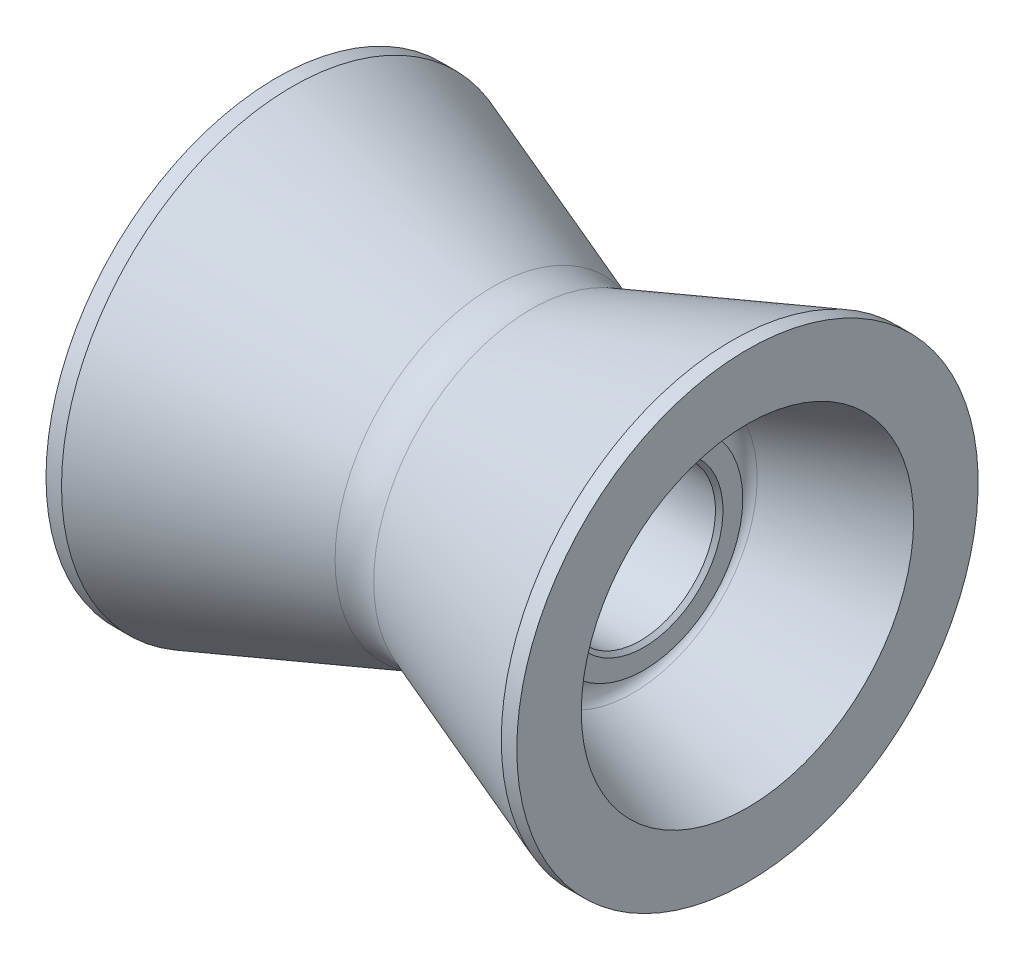
from build123d import *

# Parameters (mm, degrees)
CUT_EXTRUDE1_DEPTH = 261.839989265
CHAMFER1_SIZE      = 2
FILLET1_R          = 0.5


with BuildPart() as part:
    # Sketch1 → Revolve1 (revolve)
    with BuildSketch(Plane.XY, mode=Mode.PRIVATE) as revolve1_sk:
        with BuildLine():
            Line((-125, 122.5), (-116.767790327, 122.5))
            Line((-116.767790327, 122.5), (-10.2606043, 83.734554551))
            ThreePointArc((-10.2606043, 83.734554551), (0, 81.925333174), (10.2606043, 83.734554551))
            Line((10.2606043, 83.734554551), (116.767790327, 122.5))
            Line((116.767790327, 122.5), (125, 122.5))
            Line((125, 122.5), (125, 88.250057247))
            Line((125, 88.250057247), (64.082356705, 66.077848346))
            ThreePointArc((64.082356705, 66.077848346), (59.582843437, 58.284462756), (66.476497708, 52.5))
            Line((66.476497708, 52.5), (70, 52.5))
            Line((70, 52.5), (70, 0))
            Line((70, 0), (-70, 0))
            Line((-70, 0), (-70, 52.5))
            Line((-70, 52.5), (-66.476497708, 52.5))
            ThreePointArc((-66.476497708, 52.5), (-59.582843437, 58.284462756), (-64.082356705, 66.077848346))
            Line((-64.082356705, 66.077848346), (-125, 88.250057247))
            Line((-125, 88.250057247), (-125, 122.5))
        make_face()
    revolve(revolve1_sk.sketch.rotate(Axis((-70, 0, 0), (1, 0, 0)), 90), axis=Axis((-70, 0, 0), (1, 0, 0)))

    # Sketch2 → Cut-Extrude1 (cut, through all)
    with BuildSketch(Plane.ZY.offset(70)):
        with BuildLine():
            Line((-11, 45.4), (11, 45.4))
            Line((11, 45.4), (11, 38.457769046))
            ThreePointArc((11, 38.457769046), (0, -40), (-11, 38.457769046))
            Line((-11, 38.457769046), (-11, 45.4))
        make_face()
    extrude(amount=-CUT_EXTRUDE1_DEPTH, mode=Mode.SUBTRACT)

    # Chamfer1
    chamfer1_edges = [part.edges().sort_by_distance(p)[0] for p in [
        (70, -40, 0),
        (-70, -40, 0),
    ]]
    chamfer(chamfer1_edges, length=CHAMFER1_SIZE)

    # Fillet1
    fillet1_edges = [part.edges().sort_by_distance(p)[0] for p in [
        (0, 45.4, -11),
        (0, 45.4, 11),
    ]]
    fillet(fillet1_edges, radius=FILLET1_R)


solid = part.part
